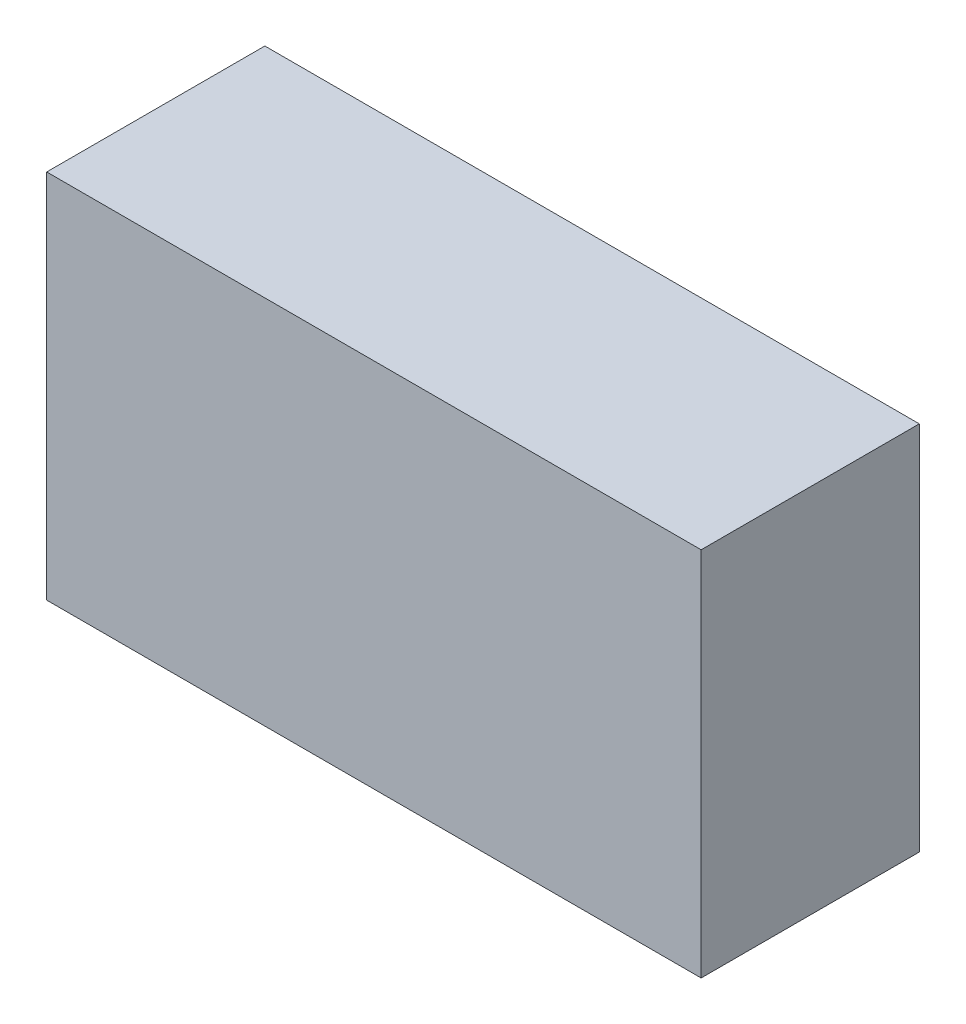
SolidWorks part; units mm, degrees
ref_plane "前视基准面" through (0, 0, 0) normal (0, 0, 1) x (1, 0, 0)
ref_plane "上视基准面" through (0, 0, 0) normal (0, 1, 0) x (1, 0, 0)
ref_plane "右视基准面" through (0, 0, 0) normal (1, 0, 0) x (0, 0, -1)
other "Configuration Table"
sketch "草图1" plane through (0, 0, 0) normal (0, 0, 1) x (1, 0, 0)
  line L0 (-150, -85) -> (150, -85)
  line L1 (150, -85) -> (150, 85)
  line L2 (150, 85) -> (-150, 85)
  line L3 (-150, 85) -> (-150, -85)
  point P0 (0, 0)
  dimension "D1" = 150
  dimension "D2" = 300
  dimension "D3" = 85
  dimension "D4" = 170
extrude "凸台-拉伸1" add sketch "草图1" against normal mid plane 100
